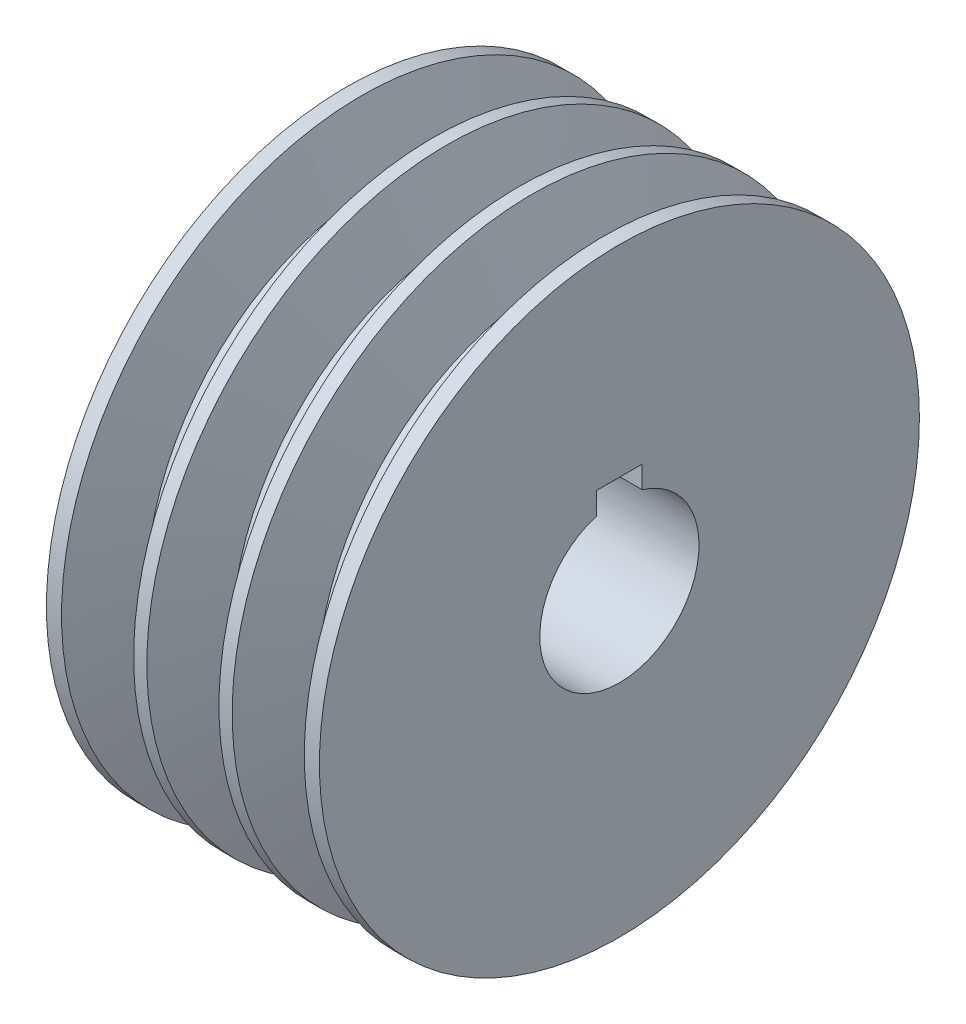
SolidWorks part; units mm, degrees
material "HT150"
ref_plane "Front Plane" through (0, 0, 0) normal (0, 0, 1) x (1, 0, 0)
ref_plane "Top Plane" through (0, 0, 0) normal (0, 1, 0) x (1, 0, 0)
ref_plane "Right Plane" through (0, 0, 0) normal (1, 0, 0) x (0, 0, -1)
sketch "Sketch1" plane through (0, 0, 0) normal (0, 0, 1) x (1, 0, 0)
  line L0 (6.1588, 41.3) -> (2.6582, 52.75)
  line L1 (2.6582, 52.75) -> (0, 52.75)
  line L2 (0, 52.75) -> (0, 14)
  line L3 (0, 14) -> (48, 14)
  line L4 (48, 14) -> (48, 52.75)
  line L5 (48, 52.75) -> (45.3418, 52.75)
  line L6 (45.3418, 52.75) -> (41.8412, 41.3)
  line L7 (41.8412, 41.3) -> (36.1612, 41.3)
  line L8 (36.1612, 41.3) -> (32.6606, 52.75)
  line L9 (32.6606, 52.75) -> (30.3406, 52.75)
  line L10 (30.3406, 52.75) -> (26.84, 41.3)
  line L11 (26.84, 41.3) -> (21.16, 41.3)
  line L12 (21.16, 41.3) -> (17.6594, 52.75)
  line L13 (17.6594, 52.75) -> (15.3394, 52.75)
  line L14 (15.3394, 52.75) -> (11.8388, 41.3)
  line L15 (11.8388, 41.3) -> (6.1588, 41.3)
  line L16 (0, 0) -> (61, 0) construction
  line L17 (8.9988, 41.3) -> (8.9988, 163.0492) construction
  line L18 (24, 41.3) -> (24, 47.1472) construction
  line L19 (39.0012, 41.3) -> (39.0012, 61.0464) construction
  point P24 (24, 14)
  dimension "D1" = 28
  dimension "D2" = 105.5
  dimension "D3" = 48
  dimension "D4" = 5.68
  dimension "D5" = 34
  dimension "D6" = 82.6
  dimension "D7" = 2.32
revolve "Revolve1" add sketch "Sketch1" angle 360 about L16
sketch "Sketch8" plane through (0, 0, 0) normal (-1, 0, 0) x (0, 0, 1)
  circle A0 centre (0, 0) radius 25
  circle A1 centre (0, 0) radius 14 construction
  circle A2 centre (0, 0) radius 14
  dimension "D1" = 50
extrude "Boss-Extrude2" add sketch "Sketch8" along normal blind 4
sketch "Sketch9" plane through (-4, 0, 0) normal (-1, 0, 0) x (0, 0, 1)
  line L0 (0, 0) -> (0, 14) construction
  line L1 (4, 17.3) -> (-4, 17.3)
  line L2 (4, 17.3) -> (4, 10.7)
  line L3 (4, 10.7) -> (-4, 10.7)
  line L4 (-4, 17.3) -> (-4, 10.7)
  line L5 (4, 17.3) -> (-4, 10.7) construction
  line L6 (4, 10.7) -> (-4, 17.3) construction
  circle A0 centre (0, 0) radius 14 construction
  point P0 (0, 14)
  dimension "D1" = 8
  dimension "D2" = 31.3
extrude "Cut-Extrude5" cut sketch "Sketch9" against normal up to next
